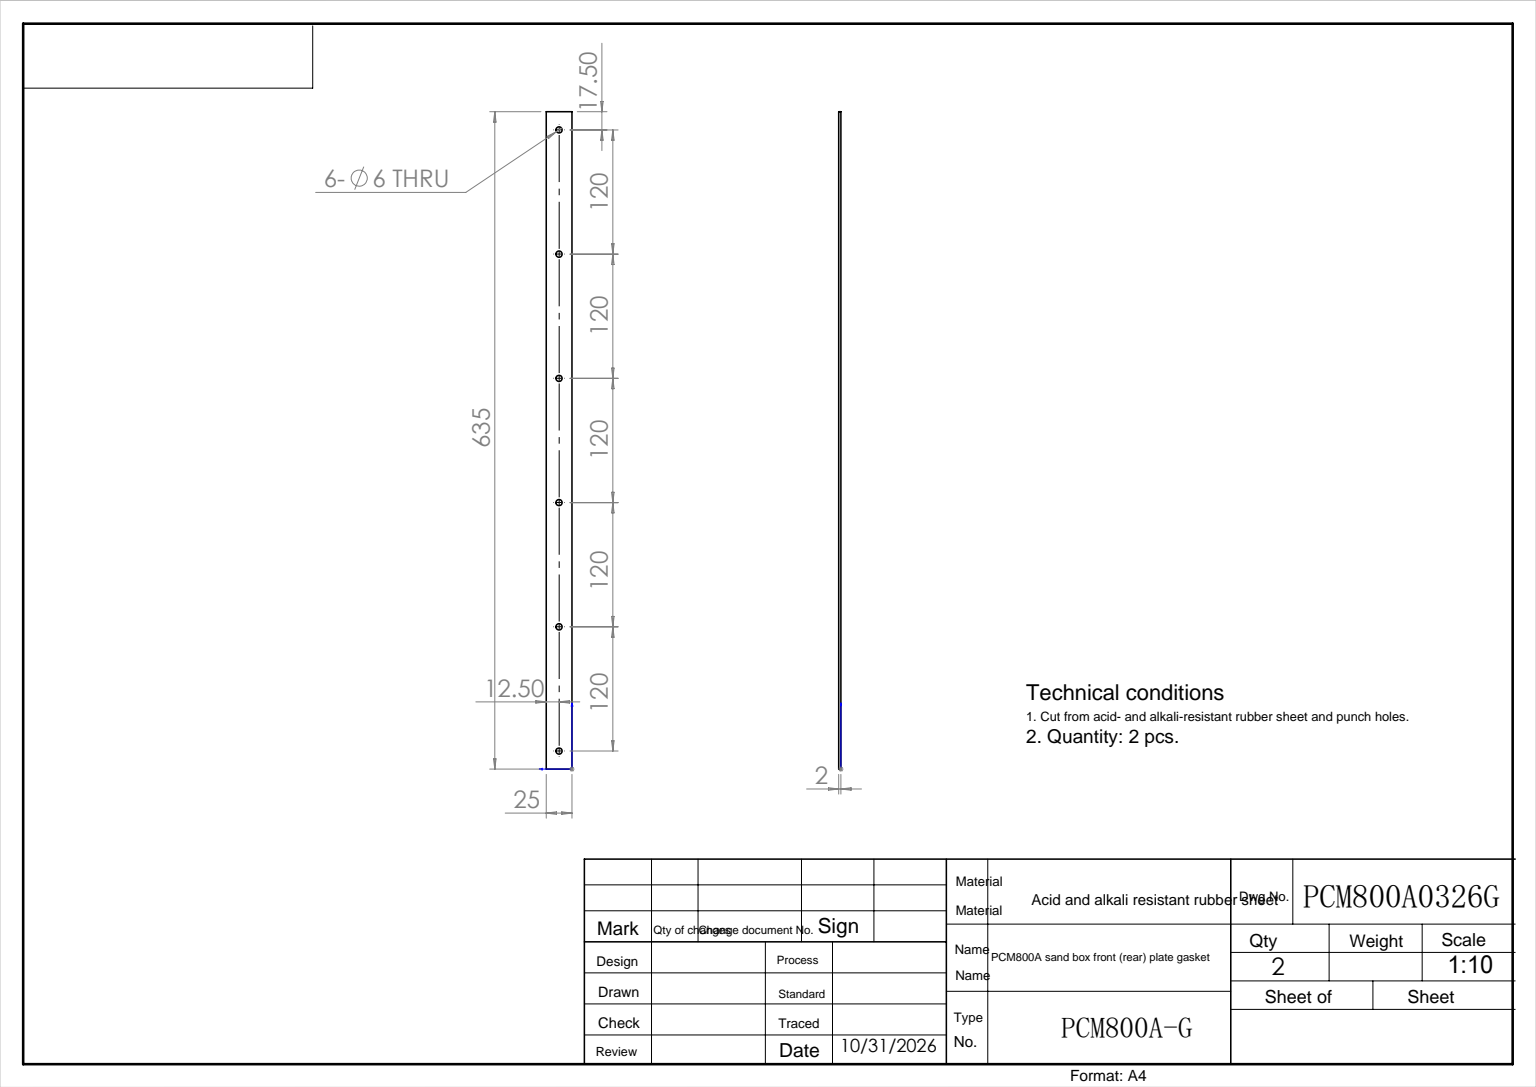
from build123d import *

# Parameters (mm, degrees)
SKETCH_1_W             = 25
SKETCH_1_H             = 635
EXTRUDE_1_DEPTH        = 2
SKETCH_3_R             = 3
CUT_EXTRUDE_1_DEPTH    = 636.495082593
PATTERN_LINEAR_1_COUNT = 6
PATTERN_LINEAR_1_PITCH = 120


with BuildPart() as part:
    # 草图1 → 拉伸1 (new body)
    with BuildSketch(Plane.XY):
        with Locations((12.5, 317.5)):
            Rectangle(SKETCH_1_W, SKETCH_1_H)
    extrude(amount=EXTRUDE_1_DEPTH)

    # 草图3 → 切除-拉伸1 (cut, through all)
    with BuildSketch(Plane.XY.offset(2)):
        with Locations((12.5, 617.5)):
            Circle(SKETCH_3_R)
    cut_extrude_1 = extrude(amount=-CUT_EXTRUDE_1_DEPTH, mode=Mode.SUBTRACT)

    # 阵列(线性)1: 切除-拉伸1 ×6
    with Locations(*[(0, -i * PATTERN_LINEAR_1_PITCH, 0) for i in range(1, PATTERN_LINEAR_1_COUNT)]):
        add(cut_extrude_1, mode=Mode.SUBTRACT)


solid = part.part
